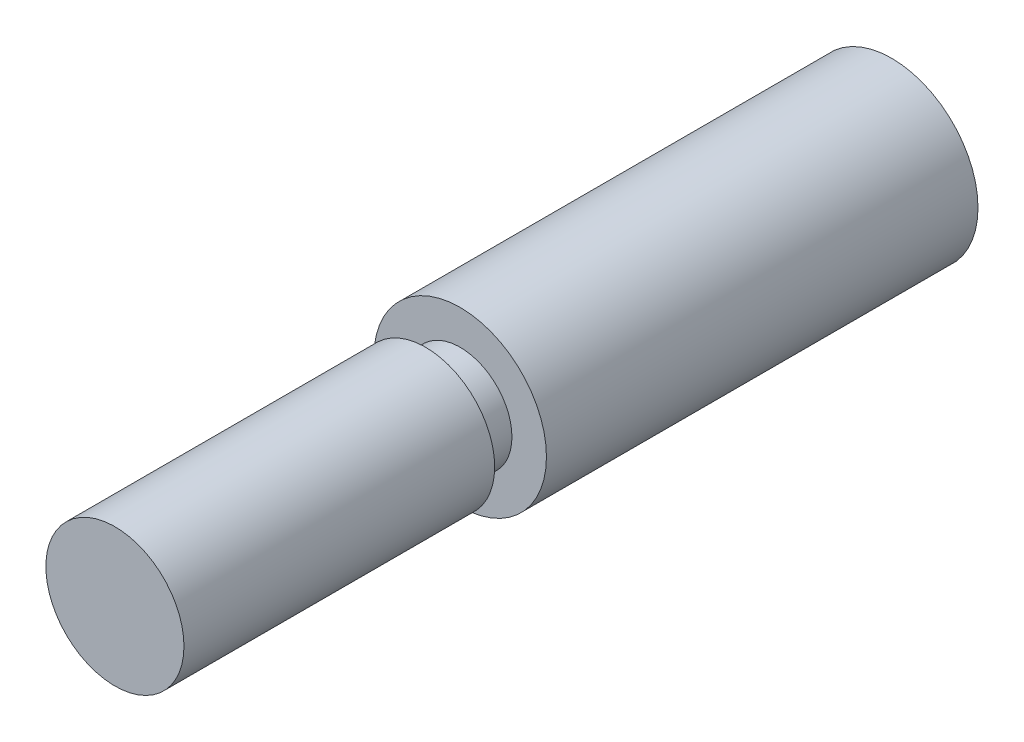
SolidWorks part; units mm, degrees
material "316L"
ref_plane "Front Plane" through (0, 0, 0) normal (0, 0, 1) x (1, 0, 0)
ref_plane "Top Plane" through (0, 0, 0) normal (0, 1, 0) x (1, 0, 0)
ref_plane "Right Plane" through (0, 0, 0) normal (1, 0, 0) x (0, 0, -1)
sketch "Sketch1" plane through (0, 0, 0) normal (0, 0, 1) x (1, 0, 0)
  circle A0 centre (0, 0) radius 5
  dimension "D1" = 10
extrude "Boss-Extrude1" add sketch "Sketch1" along normal blind 25
sketch "Sketch2" plane through (0, 0, 25) normal (0, 0, 1) x (1, 0, 0)
  circle A0 centre (0, 0) radius 4
  dimension "D1" = 8
extrude "Boss-Extrude2" add sketch "Sketch2" along normal blind 20
cosmetic thread "Cosmetic Thread1" parameters "D2"=7
sketch "Sketch3" plane through (0, 0, 25) normal (0, 0, 1) x (1, 0, 0)
  circle A0 centre (0, 0) radius 3
  dimension "D1" = 6
extrude "Cut-Extrude1" cut sketch "Sketch3" along normal blind 2 flip side to cut
